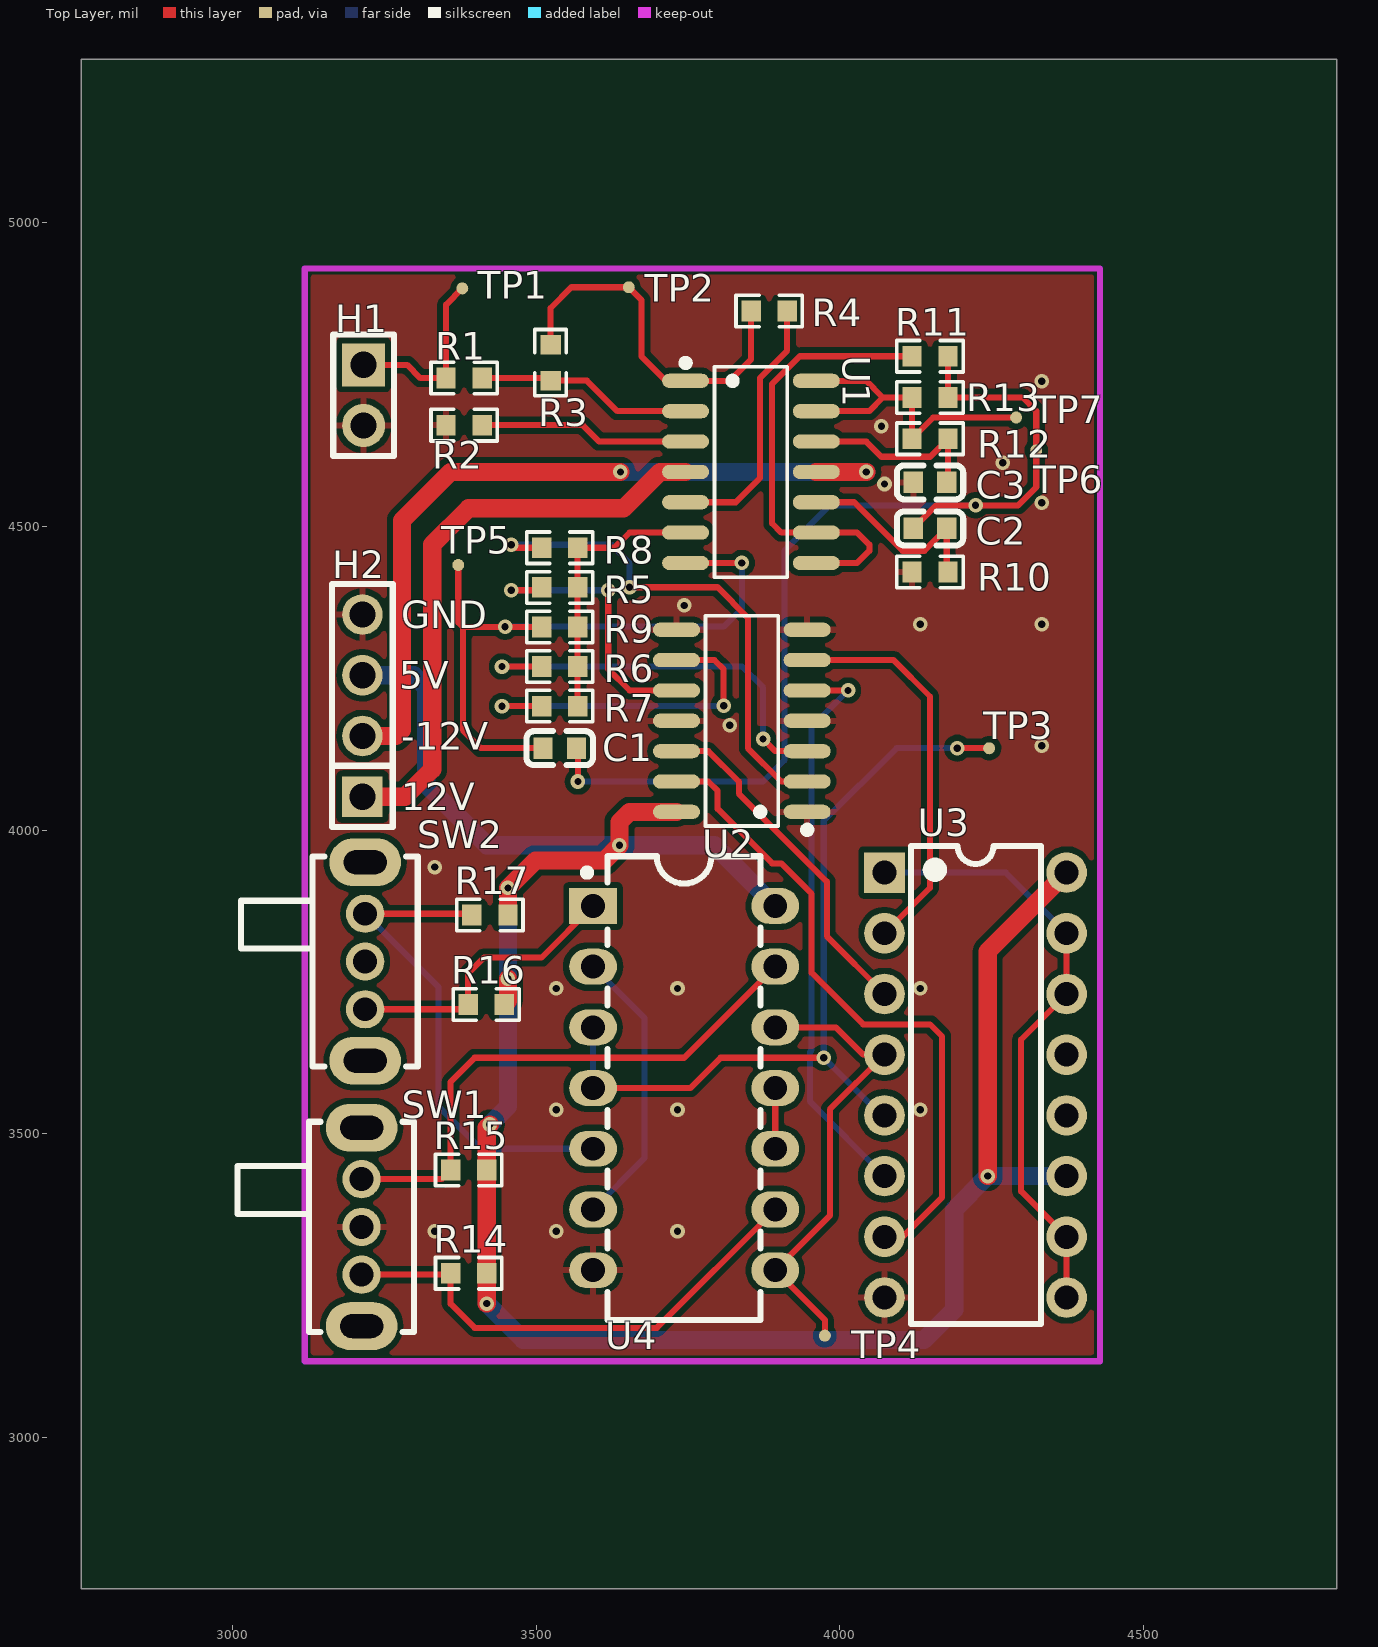
[diagram p0: Top Layer view]
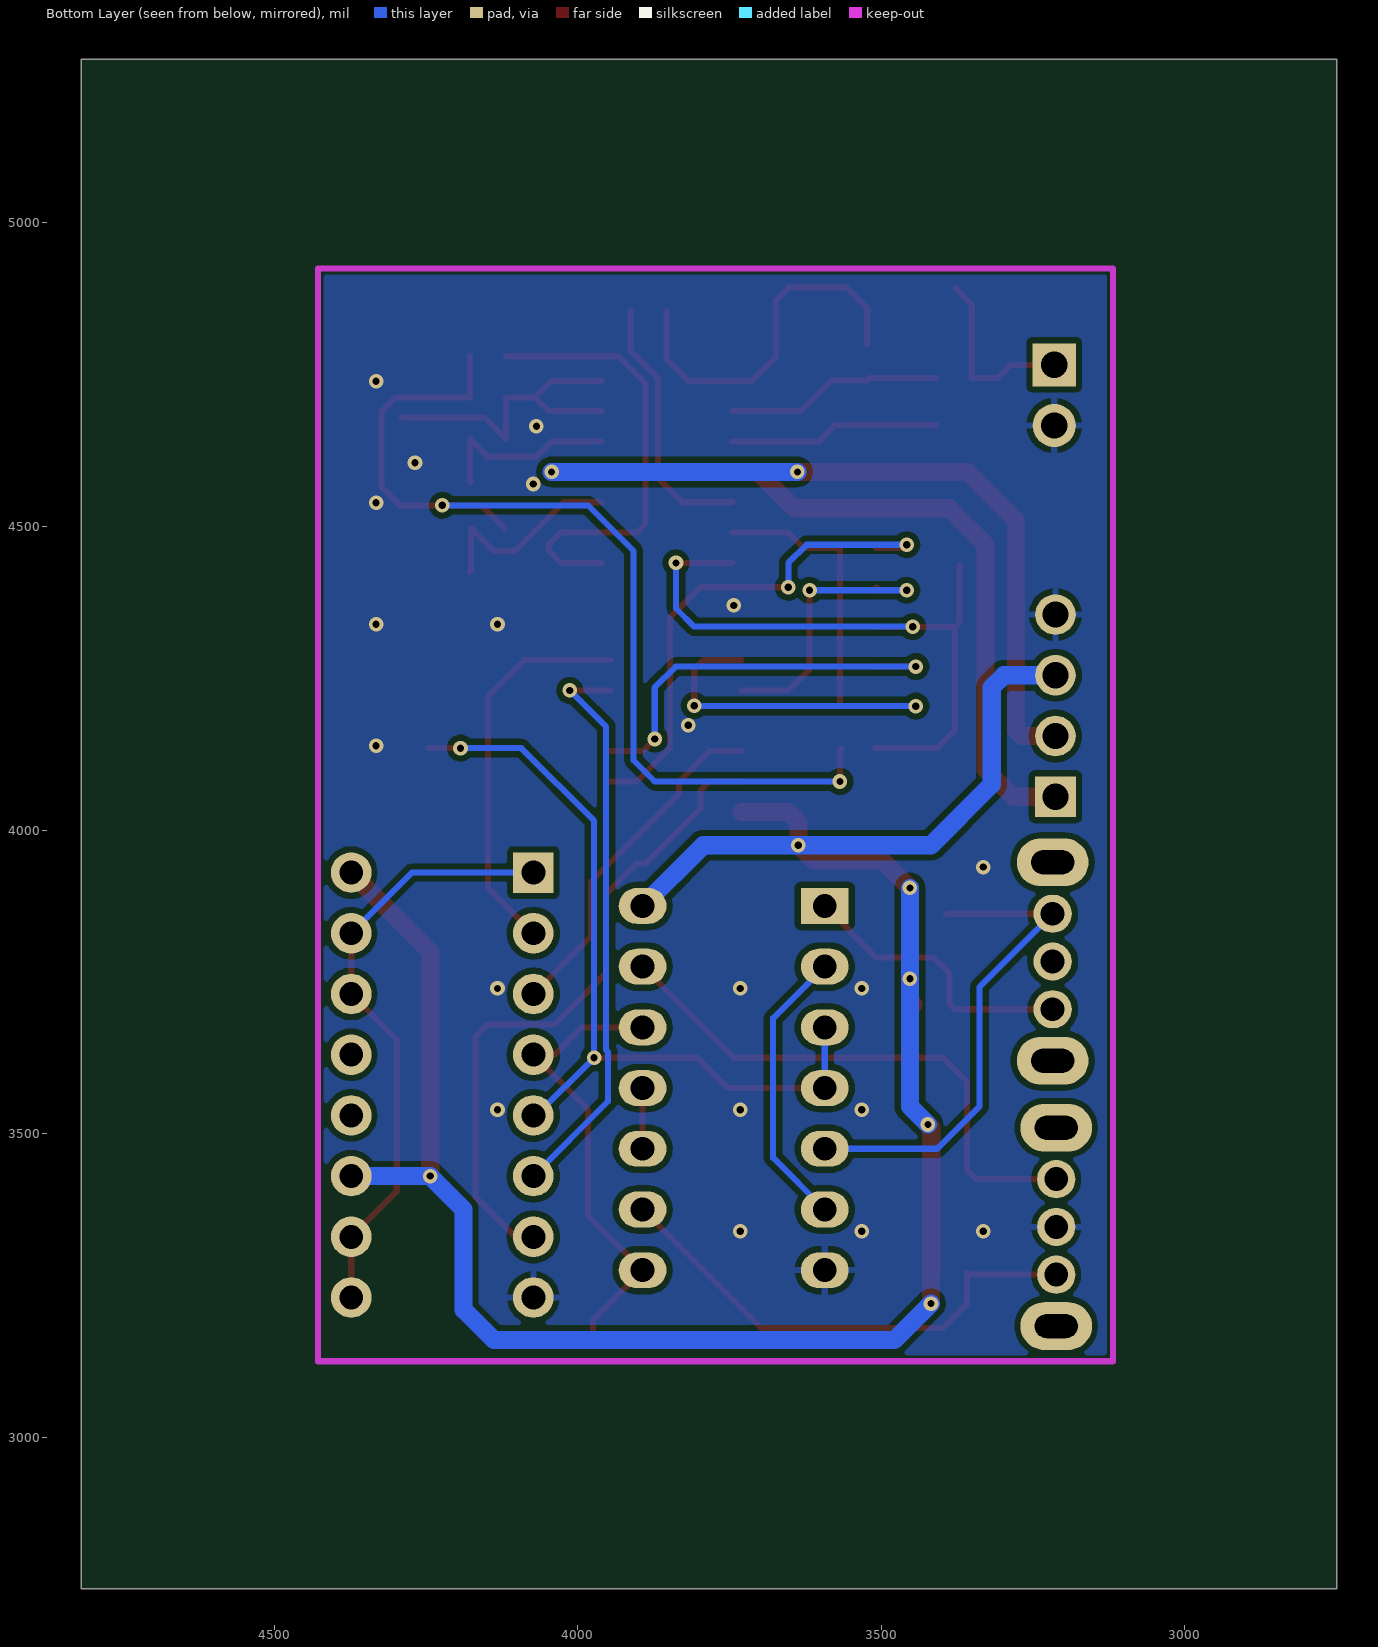
[diagram p1: Bottom Layer view, seen from below]
# Altium PCB MISC52011.pcbdoc
Units mil, origin at the board's own origin, x right, y up, seen from the top; angles counter-clockwise.
Board outline 2068.4 x 2520 mil, 2 copper layers (Top Layer, Bottom Layer), stack 62.206 mil thick; 35 components, 33 nets, 121 pads, 43 vias.

## Layer stack, top to bottom
Top Solder Mask Layer: solder mask 0.394, Dk 3.3
Top Layer: signal copper 1.379
Dielectric1: surface 59.449, FR4, Dk 4.5
Bottom Layer: signal copper 1.378
Bottom Solder Mask Layer: solder mask 0.394, Dk 3.3

## Board outline
4818.4,2750 2750,2750 2750,5270 4818.4,5270

## Design rules (kind name [scope] priority, off if disabled: settings)
BoardOutlineClearance copperThickness2oz_1 [All] p2 off: genericclearance=7.99 ignorepadtopadclearanceinfootprint=FALSE except(0: Arc-SplitContinuation Track-SplitContinuation SMDPad-SplitContinuation THPad-SplitContinuation Via-SplitContinuation Fill-SplitContinuation Region-SplitContinuation Poly-SplitContinuation Text-SplitContinuation Hole-SplitContinuation; 5.98: Arc-CutoutEdge SMDPad-CutoutEdge THPad-CutoutEdge Via-CutoutEdge Fill-CutoutEdge Region-CutoutEdge Text-CutoutEdge; 6.93: Hole-OutlineEdge Hole-CutoutEdge; 10: Poly-OutlineEdge Poly-CutoutEdge; 11.81: Arc-OutlineEdge Track-OutlineEdge SMDPad-OutlineEdge THPad-OutlineEdge Via-OutlineEdge Fill-OutlineEdge Region-OutlineEdge Text-OutlineEdge Track-CutoutEdge)
BoardOutlineClearance copperThickness1oz_1 [All] p4: genericclearance=4.02 ignorepadtopadclearanceinfootprint=FALSE except(0: Arc-SplitContinuation Track-SplitContinuation SMDPad-SplitContinuation THPad-SplitContinuation Via-SplitContinuation Fill-SplitContinuation Region-SplitContinuation Poly-SplitContinuation Text-SplitContinuation Hole-SplitContinuation; 6: SMDPad-CutoutEdge THPad-CutoutEdge Via-CutoutEdge Fill-CutoutEdge Region-CutoutEdge Text-CutoutEdge; 6.93: Hole-OutlineEdge Hole-CutoutEdge; 10: Poly-OutlineEdge Poly-CutoutEdge; 11.8: Arc-OutlineEdge Track-OutlineEdge SMDPad-OutlineEdge THPad-OutlineEdge Via-OutlineEdge Fill-OutlineEdge Region-OutlineEdge Text-OutlineEdge; 11.81: Arc-CutoutEdge Track-CutoutEdge)
Clearance copperThickness2oz [All] p1 off: gap=7.99 ignorepadtopadclearanceinfootprint=FALSE except(5.98: SMDPad-Track SMDPad-SMDPad THPad-Track SMDPad-THPad THPad-THPad Track-Via SMDPad-Via THPad-Via Via-Via Fill-Track Region-Track Fill-SMDPad Region-SMDPad Fill-THPad Region-THPad Fill-Via Region-Via Fill-Fill Fill-Region Region-Region Arc-Track Arc-SMDPad Arc-THPad Arc-Via Fill-Arc Region-Arc Arc-Arc Text-Track SMDPad-Text Text-THPad Text-Via Fill-Text Region-Text Arc-Text Text-Text; 6.93: Hole-Track Hole-SMDPad Hole-THPad Hole-Via Fill-Hole Region-Hole Hole-Arc Hole-Text; 10: Poly-Track Poly-SMDPad Poly-THPad Poly-Via Poly-Fill Poly-Region Poly-Poly Poly-Arc Poly-Text Poly-Hole)
Clearance copperThickness1oz [All] p3: gap=4.02 ignorepadtopadclearanceinfootprint=FALSE except(5.98: SMDPad-Track SMDPad-SMDPad THPad-Track SMDPad-THPad THPad-THPad Track-Via SMDPad-Via THPad-Via Via-Via Fill-Track Region-Track Fill-SMDPad Region-SMDPad Fill-THPad Region-THPad Fill-Via Region-Via Fill-Fill Fill-Region Region-Region; 6: Arc-Track Arc-SMDPad Arc-THPad Arc-Via Fill-Arc Region-Arc Arc-Arc Text-Track SMDPad-Text Text-THPad Text-Via Fill-Text Region-Text Arc-Text Text-Text; 6.93: Hole-Track Hole-SMDPad Hole-THPad Hole-Via Fill-Hole Region-Hole Hole-Arc Hole-Text; 10: Poly-Track Poly-SMDPad Poly-THPad Poly-Via Poly-Fill Poly-Region Poly-Poly Poly-Arc Poly-Text Poly-Hole)
DiffPairsRouting differentialPair [All] p1: maxlimit=6 minlimit=6 mostfreqgap=6 toplayer_minwidth=5 toplayer_prefwidth=10 toplayer_maxwidth=100 toplayer_mingap=6 toplayer_prefgap=6 toplayer_maxgap=6 bottomlayer_minwidth=5 bottomlayer_prefwidth=10 bottomlayer_maxwidth=100 bottomlayer_mingap=6 bottomlayer_prefgap=6 bottomlayer_maxgap=6 maxuncoupledlength=10
HoleToHoleClearance otherClearance [All] p1: gap=11.81 allowstackedmicrovias=TRUE
Length netLength [All] p1: minlimit=0 maxlimit=0
MatchedLengths netLengthTolerance [All] p1: tolerance=1000
PasteMaskExpansion pasteMaskExpansion [All] p1: expansion=0
PlaneConnect innerPlane [All] p1: planeconnectstyle=Relief reliefexpansion=20 reliefentries=4 reliefconductorwidth=10 reliefairgap=10
PolygonConnect copperRegion [(InNet('GND'))] p1: connectstyle=Relief reliefconductorwidth=10 reliefentries=4 polygonreliefangle="90 Angle" airgapwidth=10 via.connectstyle=Relief via.reliefconductorwidth=10 via.reliefentries=4 via.polygonreliefangle="90 Angle" via.airgapwidth=10
RoutingVias viaSize [All] p1: holewidth=12.01 width=24.02 viastyle="Through Hole" minholewidth=11.81 minwidth=19.68 maxholewidth=248.03 maxwidth=393.7
SolderMaskExpansion solderMaskExpansion [IsVia] p1: expansion=-1000 istentingtop=TRUE
SolderMaskExpansion solderMaskExpansion [All] p2: expansion=2 istentingtop=FALSE
Width copperThickness2oz_2 [All] p1 off: maxlimit=100 minlimit=8 preferedwidth=10
Width copperThickness1oz_2 [All] p2: maxlimit=100 minlimit=5 preferedwidth=10

## Components (designator, comment, footprint, x,y, rotation, side; value= is the part's Value field where it differs from the comment)
C1 "150nF" C0603 3538.4,4135 r0 top
C2 "150nF" C0603 4148.4,4496.89 r0 top
C3 "20nF" C0603 4148.4,4572.73 r0 top
H1 "" HDR-TH_2P-P2.54-V-M-1 3215.37,4716.4 r270 top
H2 "" HDR-TH_4P-P2.54-V-M 3213.4,4205 r90 top
R1 "120K" R0603 3380.93,4744.62 r0 top
R2 "110K" R0603 3380.93,4666.92 r0 top
R3 "1.2M" R0603 3523.4,4770 r90 top
R4 "10K" R0603 3883.4,4855 r0 top
R5 "80K" R0603 3538.4,4399.79 r0 top
R6 "40K" R0603 3538.4,4269.37 r0 top
R7 "20K" R0603 3538.4,4204.16 r0 top
R8 "10K" R0603 3538.4,4465 r0 top
R9 "160K" R0603 3538.4,4334.58 r0 top
R10 "15K" R0603 4148.4,4425 r0 top
R11 "15K" R0603 4148.4,4780.51 r0 top
R12 "1.5K" R0603 4148.4,4644.62 r0 top
R13 "1.5K" R0603 4148.4,4712.57 r180 top
R14 "1K" R0603 3388.4,3270 r0 top
R15 "1K" R0603 3388.4,3440 r0 top
R16 "1K" R0603 3417.34,3712.79 r0 top
R17 "1K" R0603 3423.4,3860 r0 top
SW1 "" 拨动开关_侧 3212.1,3346.3 r270 top
SW2 "" 拨动开关_侧 3218,3783.5 r270 top
TP1 "" Test-Point-0.5mm 3377.97,4892.29 r0 top
TP2 "" Test-Point-0.5mm 3652.24,4894.14 r0 top
TP3 "" Test-Point-0.5mm 4245.81,4134.73 r0 top
TP4 "" Test-Point-0.5mm 3975.18,3167.31 r0 top
TP5 "" Test-Point-0.5mm 3371.26,4436.66 r0 top
TP6 "" Test-Point-0.5mm 4323.35,4625.51 r0 top
TP7 "" Test-Point-0.5mm 4290.22,4679.62 r0 top
U1 "LM324ADR" SOP-14_L8.6-W3.9-P1.27-LS6.0-BL 3853.4,4590 r270 top
U2 "CD4066BD" SOP-14_L8.6-W3.9-P1.27-LS6.0-BL 3838.4,4180 r90 top
U3 "NTE74193" PDIP-16_L19.7-W6.6-P2.54-LS7.6-BL 4223.4,3580 r270 top
U4 "SN7400N" PDIP-14_L19.3-W6.4-P2.54-LS7.9-BL-1 3743.4,3575 r270 top

## Footprints (in the part's own frame and the unit in brackets; to place one, negate y for a bottom-side part, rotate by r counter-clockwise, add the part's x,y. Pads: shape width x height; smd on the part's side, far side on the other; paste and mask are expansions set on the pad)
C0603 [mm]
  rect 0.8x0.9 smd: 1(-0.7,0) 2(0.7,0)
  silkscreen extent -1.39,-0.71 1.39,0.71
HDR-TH_2P-P2.54-V-M-1 [mm]
  rect 1.8x1.8 hole 1.1: 1(-1.27,0)
  round 1.8 hole 1.1: 2(1.27,0)
  silkscreen extent -2.54,-1.27 2.54,1.27
HDR-TH_4P-P2.54-V-M [mm]
  rect 1.7x1.7 hole 1.1: 1(-3.81,0)
  round 1.7 hole 1.1: 2(-1.27,0) 3(1.27,0) 4(3.81,0)
  silkscreen extent -5.08,-1.27 5.08,1.27
PDIP-14_L19.3-W6.4-P2.54-LS7.9-BL-1 [mm]
  rect 1.5x2 hole 1: 1(-7.62,-3.81)
  oval 1.5x2 hole 1: 2(-5.08,-3.81) 3(-2.54,-3.81) 4(0,-3.81) 5(2.54,-3.81) 6(5.08,-3.81) 7(7.62,-3.81)
  oval 1.5x2 hole 1 copper offset 0,0: 8(7.62,3.81) 9(5.08,3.81) 10(2.54,3.81) 11(0,3.81) 12(-2.54,3.81) 13(-5.08,3.81) 14(-7.62,3.81)
  silkscreen extent -9.7,-4.21 9.7,3.2
PDIP-16_L19.7-W6.6-P2.54-LS7.6-BL [mm]
  rect 1.7x1.7 hole 1: 1(-8.89,-3.81)
  round 1.7 hole 1: 2(-6.35,-3.81) 3(-3.81,-3.81) 4(-1.27,-3.81) 5(1.27,-3.81) 6(3.81,-3.81) 7(6.35,-3.81) 8(8.89,-3.81) 9(8.89,3.81) 10(6.35,3.81) 11(3.81,3.81) 12(1.27,3.81) 13(-1.27,3.81) 14(-3.81,3.81) 15(-6.35,3.81) 16(-8.89,3.81)
  silkscreen extent -10,-2.7 10,2.73
R0603 [mil]
  rect 31.75x34.02 smd paste-3937.01 mask+2: 1(-29.66,0) 2(29.66,0)
  silkscreen extent -55,-26 55,26
SOP-14_L8.6-W3.9-P1.27-LS6.0-BL [mm]
  oval 0.595x1.968 smd: 1(-3.81,-2.734) 2(-2.54,-2.734) 3(-1.27,-2.734) 4(0,-2.734) 5(1.27,-2.734) 6(2.54,-2.734) 7(3.81,-2.734) 8(3.81,2.734) 9(2.54,2.734) 10(1.27,2.734) 11(0,2.734) 12(-1.27,2.734) 13(-2.54,2.734) 14(-3.81,2.734)
  silkscreen extent -4.71,-2.88 4.4,1.52
Test-Point-0.5mm [mm]
  round 0.5 smd: 1(0,0)
拨动开关_侧 [mil]
  round 63 hole 39.4 paste+0 mask+2: 1(-78.7,0) 2(0,0) 3(78.7,0)
  oval 78.7x118.1 hole 39.4 slot 70.9 at 90 deg paste+0 mask+2: 4(163.4,0) 5(-163.4,0)
  silkscreen extent -173,-205 173,87

## Via types
v1: diameter 24.02, hole 12, Top Layer to Bottom Layer, 43 vias

## Nets (pads, with @x,y where several pads share a name; then routed paths per layer and width w, separated by ;. In a path a pad name is that pad's centre, name@x,y a point inside that pad or via, vN(x,y) a via of type N, cw(c..) or ccw(c..) an arc to the next point about the centre after c; other vN are vias at no path point)
5V: H2.3 R14.2 R15.2 R16.2 R17.2 U2.14 U3.11 U3.16 U4.14 | length 3814.1
  Top Layer w30: v1(3418.4,3220) 3418.4,3269.66 R14.2 R15.2 3418.06,3509.66 v1(3423.4,3515) ; R16.2 3453.06,3718.85 v1(3453.06,3755) ; R17.2 v1(3453.06,3904.66) 3498.4,3950 3611.83,3950 v1(3636.83,3975) 3636.83,4013.43 3653.4,4030 U2.14 ; v1(4243.4,3430) 4243.4,3800 U3.16
  Bottom Layer w30: H2.3 3298.4,4255 3318.4,4235 3318.4,4075 3418.4,3975 v1(3636.83,3975) 3793.4,3975 U4.14 ; v1(3418.4,3220) 3478.4,3160 4138.4,3160 4188.4,3210 4188.4,3375 v1(4243.4,3430) U3.11 ; v1(3423.4,3515) 3453.06,3544.66 v1(3453.06,3755) v1(3453.06,3904.66)
12V: H2.1 U1.4 | length 970.7
  Top Layer w30: H2.1 3283.4,4055 3328.4,4100 3328.4,4470 3388.4,4530 3643.4,4530 3703.4,4590 U1.4
$1N1: H1.1 R1.1 TP1.1 | length 303.6
  Top Layer w10: H1.1 3287,4766.4 3308.78,4744.62 R1.1 3351.27,4865.58 TP1.1
$1N3: R1.2 R3.1 U1.2 | length 357.8
  Top Layer w10: R1.2 3519.12,4744.62 R3.1 3583.06,4740.34 3633.4,4690 U1.2
$1N8: R4.2 U1.5 | length 432.7
  Top Layer w10: U1.5 3828.4,4540 3868.4,4580 3868.4,4745 3913.06,4789.66 R4.2
$1N9: R3.2 R4.1 TP2.1 U1.1 | length 617.4
  Top Layer w10: R3.2 3523.4,4860 3557.54,4894.14 TP2.1 3673.4,4872.98 3673.4,4780 3713.4,4740 U1.1 3818.4,4740 3853.74,4775.34 R4.1
$1N11: R5.1 U2.10 | length 469.2
  Top Layer w10: v1(3458.4,4395) 3503.95,4395 R5.1 ; v1(3618.4,4395) 3618.4,4265 3653.4,4230 U2.10
  Bottom Layer w10: v1(3458.4,4395) v1(3618.4,4395)
$1N12: R6.1 U2.3 | length 675.5
  Top Layer w10: v1(3443.4,4269.37) R6.1 ; v1(3873.4,4150) 3893.4,4130 U2.3
  Bottom Layer w10: v1(3443.4,4269.37) 3839.03,4269.37 3873.4,4235 v1(3873.4,4150)
$1N13: R7.1 U2.9 | length 574.5
  Top Layer w10: v1(3443.4,4204.16) R7.1 ; U2.9 3793.4,4280 3808.4,4265 v1(3808.4,4205)
  Bottom Layer w10: v1(3443.4,4204.16) 3807.56,4204.16 v1(3808.4,4205)
$1N14: R8.1 U2.2 | length 851
  Top Layer w10: v1(3458.4,4470) 3463.4,4465 R8.1 ; v1(3653.4,4400) 3798.4,4400 3848.4,4350 3848.4,4135 3903.4,4080 U2.2
  Bottom Layer w10: v1(3458.4,4470) 3623.4,4470 3653.4,4440 v1(3653.4,4400)
$1N16: U2.12 U3.3 | length 572.8
  Top Layer w10: U2.12 3783.4,4130 3833.4,4080 3833.4,4060 3978.4,3915 3978.4,3825 U3.3
$1N17: U2.6 U3.2 | length 648.3
  Top Layer w10: U2.6 4088.4,4280 4148.4,4220 4148.4,3905 U3.2
$1N18: U2.5 U3.6 | length 944.4
  Top Layer w10: U2.5 v1(4013.4,4230)
  Bottom Layer w10: v1(4013.4,4230) 3953.4,4170 3953.4,3637.52 3950.41,3634.52 3950.41,3552.99 U3.6
$1N19: U2.13 U3.7 | length 1092.2
  Top Layer w10: U2.13 3783.4,4080 3798.4,4065 3798.4,4035.01 3888.41,3945 3903.4,3945 3953.4,3895 3953.4,3765 4038.4,3680 4148.4,3680 4168.4,3660 4168.4,3395 4103.4,3330 U3.7
$1N21: U3.1 U3.9 U3.10 U3.14 U3.15 | length 1003.6
  Top Layer w10: U3.9 U3.10 4298.4,3405 4298.4,3655 U3.14 U3.15
  Bottom Layer w10: U3.1 4273.4,3930 U3.15
$1N22: TP4.1 U3.4 U4.8 U4.12 | length 769.8
  Top Layer w10: U4.12 3993.4,3675 4038.4,3630 U3.4 3983.4,3540 3983.4,3365 U4.8 3975.18,3193.22 TP4.1
$1N23: TP3.1 U3.5 U4.3 U4.4 | length 1352.3
  Top Layer w10: U4.4 3753.4,3575 3803.4,3625 v1(3973.4,3625) ; v1(4193.4,4135) 4245.54,4135 TP3.1
  Bottom Layer w10: U4.4 U4.3 ; U3.5 4068.4,3530 v1(3973.4,3625) 3973.4,4015 4093.4,4135 v1(4193.4,4135)
$1N26: C1.1 R9.1 TP5.1 U1.7 | length 1119.5
  Top Layer w10: TP5.1 3371.26,4342.14 3378.82,4334.58 ; R9.1 3378.82,4334.58 ; C1.1 3408.4,4135 3378.82,4164.58 3378.82,4334.58 ; U1.7 v1(3838.4,4440)
  Bottom Layer w10: v1(3448.4,4335) 3808.4,4335 3838.4,4365 v1(3838.4,4440)
$1N27: R5.2 R6.2 R7.2 R8.2 R9.2 U1.6 | length 448.9
  Top Layer w10: R7.2 R6.2 R9.2 R5.2 R8.2 3628.4,4465 3653.4,4490 U1.6
$1N29: C2.2 R10.2 U1.10 | length 336.1
  Top Layer w10: U1.10 4023.4,4540 4103.4,4460 4139.07,4460 C2.2 4175.96,4427.1 R10.2
$1N32: R11.1 U1.8 U1.9 | length 759.3
  Top Layer w10: U1.8 4028.4,4440 4048.4,4460 4048.4,4470 4028.4,4490 U1.9 3903.4,4490 3888.4,4505 3888.4,4735 3933.91,4780.51 R11.1
$1N33: C1.2 C2.1 R11.2 R13.1 TP6.1 | length 1679.9
  Top Layer w10: C1.2 3568.4,4132.56 v1(3568.4,4080) ; C2.1 4158.95,4535 v1(4223.4,4535) 4293.4,4535 4323.35,4564.95 TP6.1 4323.35,4690.05 4300.83,4712.57 R13.1 R11.2
  Bottom Layer w10: v1(3568.4,4080) 3873.4,4080 3908.4,4115 3908.4,4460 3983.4,4535 v1(4223.4,4535)
$1N35: R12.1 R13.2 TP7.1 U1.13 U1.14 | length 542.1
  Top Layer w10: U1.13 4048.26,4690 4070.83,4712.57 ; U1.14 4043.4,4740 4070.83,4712.57 ; TP7.1 4153.74,4679.62 R12.1 R13.2 4070.83,4712.57
$1N36: C3.2 R12.2 U1.12 | length 312.4
  Top Layer w10: U1.12 4043.4,4640 4068.4,4615 4148.44,4615 R12.2 4178.06,4574.83 C3.2
$1N38: U4.10 U4.11 | length 100
  Top Layer w10: U4.10 U4.11
$1N39: R15.1 SW1.1 U4.13 | length 911.4
  Top Layer w10: SW1.1 3343.74,3425 R15.1 3358.74,3585.34 3398.4,3625 3743.4,3625 U4.13
$1N41: R14.1 SW1.3 U4.9 | length 829.8
  Top Layer w10: SW1.3 3356.34,3267.6 R14.1 3358.74,3219.66 3398.4,3180 3698.4,3180 U4.9
$1N43: R16.1 SW2.3 U4.1 | length 476.1
  Top Layer w10: SW2.3 3379.69,3704.8 R16.1 3387.68,3764.28 3413.4,3790 3508.41,3790 U4.1
$1N44: R17.1 SW2.1 U4.5 | length 827.7
  Top Layer w10: SW2.1 3391.54,3862.2 R17.1
  Bottom Layer w10: SW2.1 3338.4,3741.8 3338.4,3545 3408.4,3475 U4.5
$1N45: U4.2 U4.6 | length 470.4
  Bottom Layer w10: U4.6 3678.4,3460 3678.4,3690 U4.2
$1N52: R2.2 U1.3 | length 346.3
  Top Layer w10: R2.2 3576.48,4666.92 3603.4,4640 U1.3
-12V: H2.2 U1.11 | length 1294.6
  Top Layer w30: H2.2 3268.4,4155 3278.4,4165 3278.4,4510 3358.4,4590 v1(3638.4,4590) ; U1.11 v1(4043.4,4590)
  Bottom Layer w30: v1(3638.4,4590) v1(4043.4,4590)
GND: C3.1 H1.2 H2.4 R2.1 R10.1 SW1.2 U2.1 U2.4 U2.7 U2.8 U2.11 U3.8 U4.7
  other v1: 3332.5,3339.1 3532.5,3339.1 3732.5,3339.1 3532.5,3539.1 3732.5,3539.1 4132.5,3539.1 3532.5,3739.1 3732.5,3739.1 4132.5,3739.1 3332.5,3939.1 4332.5,4139.1 3818.3,4172.47 4132.5,4339.1 4332.5,4339.1 3743.4,4370 4332.5,4539.1 4073.4,4570 4268.4,4605 4068.4,4665 4332.5,4739.1
pads on no net: SW1.4 SW1.5 SW2.2 SW2.4 SW2.5 U3.12 U3.13

## Polygon pours and split planes (outlines as drawn)
GND on Top Layer (solid, remove dead copper, pour order 0): 3028.4,5000 3028.4,3040 4568.4,3040 4568.4,5000
GND on Bottom Layer (solid, remove dead copper, pour order 2): 3043.4,5020 3043.4,3000 4548.4,3000 4548.4,5020

## Keep-outs
Board Outline Layer:
  lines w10: 3118.4,3125 3118.4,4925 4428.4,4925 4428.4,3125 3118.4,3125

## Silkscreen, mask and mechanical layers (free items; w line width, h text height)
Top Silkscreen Layer:
  text "GND" at 3277.4,4332.5 h45
  text "5V" at 3274.28,4232.5 h45
  text "-12V" at 3277.35,4131.96 h45
  text "12V" at 3277.35,4032.5 h45